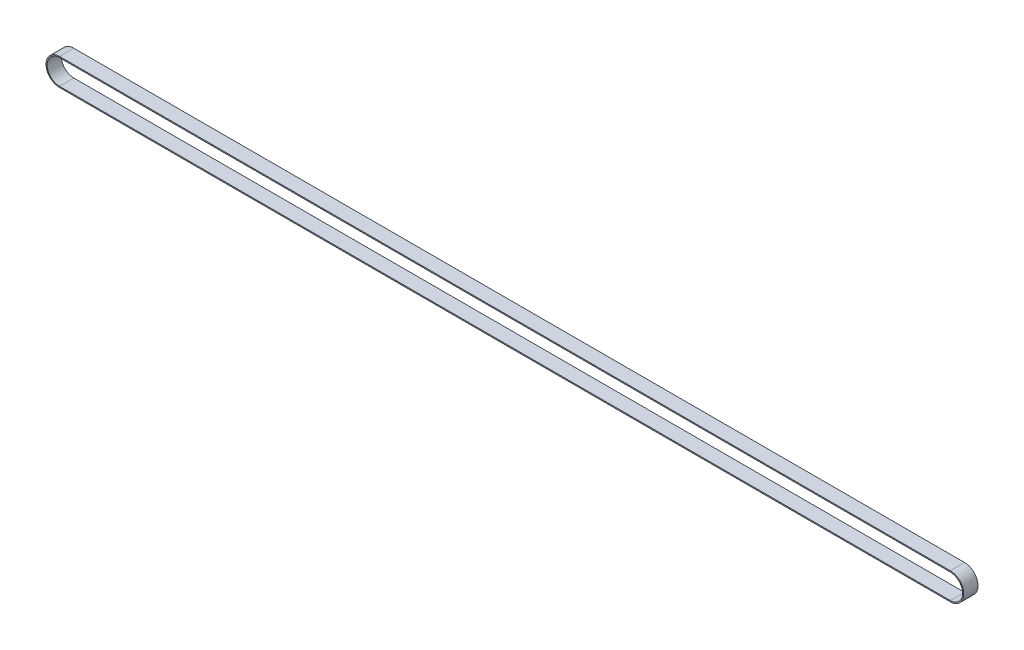
from build123d import *

# Parameters (mm, degrees)
EXTRUDE_1_DEPTH = 7.5


with BuildPart() as part:
    # 草图1 → 凸台-拉伸1 (new, symmetric)
    with BuildSketch(Plane.XY):
        with BuildLine():
            Line((0, 14.17), (937, 14.17))
            ThreePointArc((937, 14.17), (951.17, 0), (937, -14.17))
            Line((937, -14.17), (0, -14.17))
            ThreePointArc((0, -14.17), (-14.17, 0), (0, 14.17))
        make_face()
        with BuildLine():
            Line((0, 12.99), (937, 12.99))
            ThreePointArc((937, 12.99), (949.99, 0), (937, -12.99))
            Line((937, -12.99), (0, -12.99))
            ThreePointArc((0, -12.99), (-12.99, 0), (0, 12.99))
        make_face(mode=Mode.SUBTRACT)
    extrude(amount=EXTRUDE_1_DEPTH, both=True)


solid = part.part
